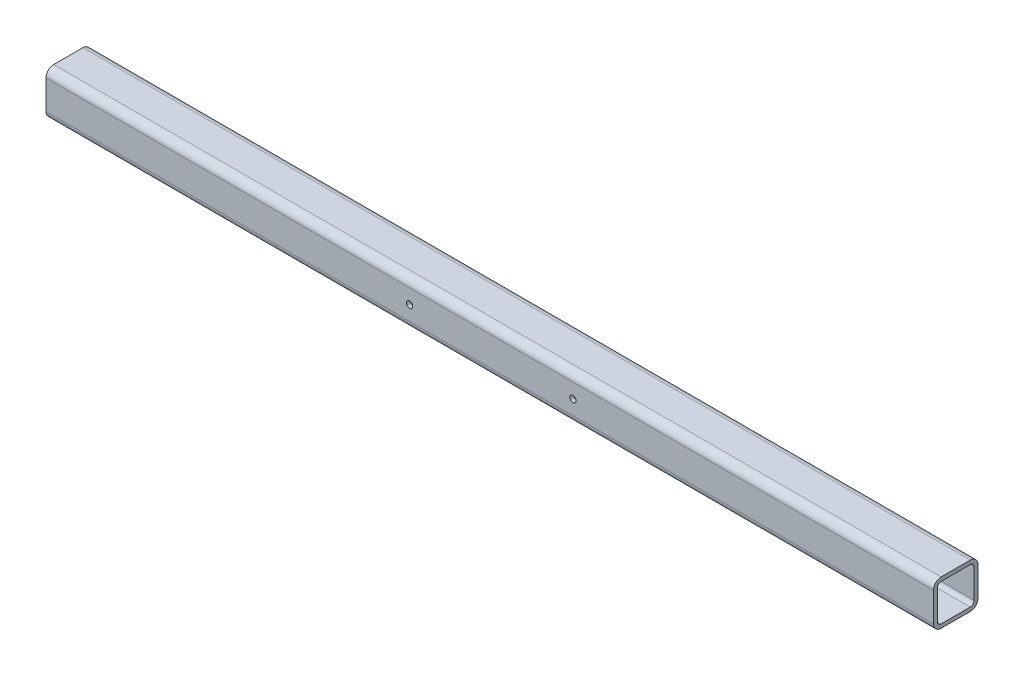
from build123d import *

# Parameters (mm, degrees)
MEMBER_1_DEPTH     = 598
HOLE_WIZARD_M5_1_D = 4.2


with BuildPart() as part:
    # Sketch1 → Member 1 (new body)
    with BuildSketch(Plane(origin=(0, 0, 0), x_dir=(0, 0, -1), z_dir=(1, 0, 0))):
        with BuildLine():
            Line((-9.8, -15), (9.8, -15))
            ThreePointArc((9.8, -15), (13.476955262, -13.476955262), (15, -9.8))
            Line((15, -9.8), (15, 9.8))
            ThreePointArc((15, 9.8), (13.476955262, 13.476955262), (9.8, 15))
            Line((9.8, 15), (-9.8, 15))
            ThreePointArc((-9.8, 15), (-13.476955262, 13.476955262), (-15, 9.8))
            Line((-15, 9.8), (-15, -9.8))
            ThreePointArc((-15, -9.8), (-13.476955262, -13.476955262), (-9.8, -15))
        make_face()
        with BuildLine():
            Line((-9.8, -12.4), (9.8, -12.4))
            ThreePointArc((9.8, -12.4), (11.638477631, -11.638477631), (12.4, -9.8))
            Line((12.4, -9.8), (12.4, 9.8))
            ThreePointArc((12.4, 9.8), (11.638477631, 11.638477631), (9.8, 12.4))
            Line((9.8, 12.4), (-9.8, 12.4))
            ThreePointArc((-9.8, 12.4), (-11.638477631, 11.638477631), (-12.4, 9.8))
            Line((-12.4, 9.8), (-12.4, -9.8))
            ThreePointArc((-12.4, -9.8), (-11.638477631, -11.638477631), (-9.8, -12.4))
        make_face(mode=Mode.SUBTRACT)
    extrude(amount=MEMBER_1_DEPTH)

    # M5 螺纹孔1 (through all)
    with Locations(Plane.XY.offset(15)):
        with Locations((355.000000009, 0), (245.000000009, 0)):
            Hole(HOLE_WIZARD_M5_1_D / 2)


solid = part.part
